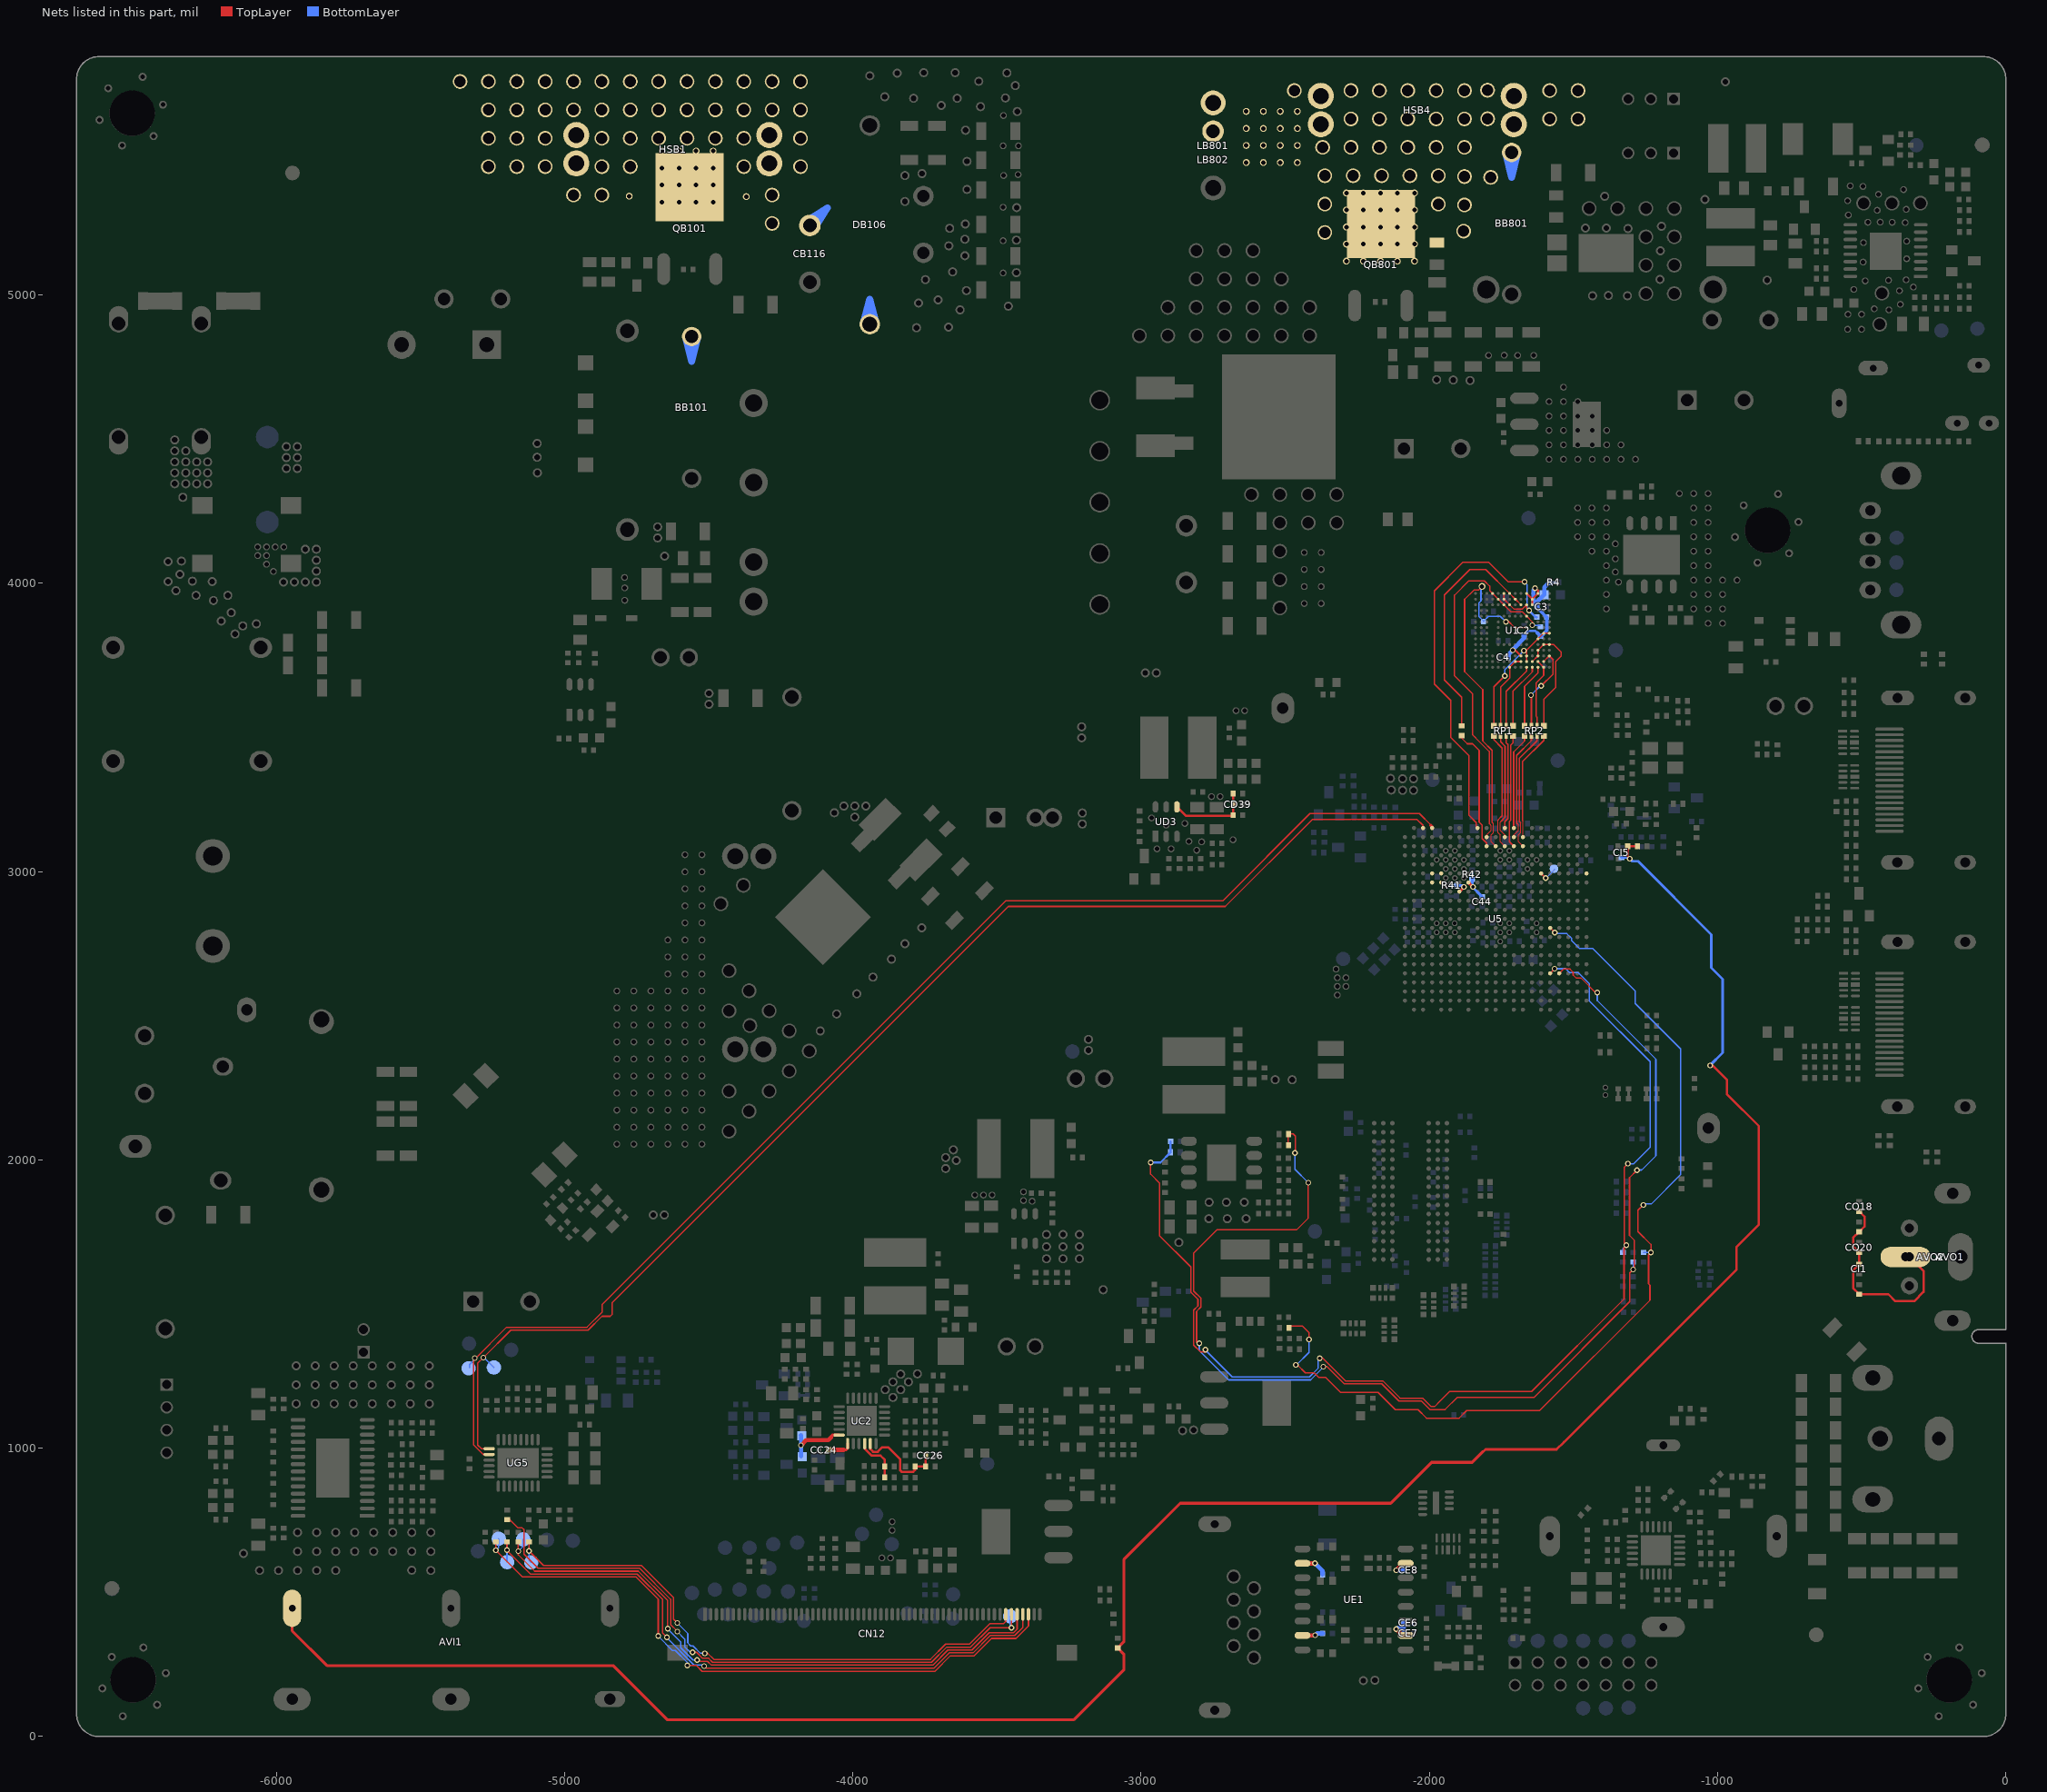
[diagram p0: the nets of this part, all layers, seen from the top]
# Altium PCB MISC84395.PcbDoc (part 12 of 26)
Units mil, origin at the board's own origin, x right, y up, seen from the top; angles counter-clockwise.
Board outline 6692.91 x 5826.77 mil, 2 copper layers (TopLayer, BottomLayer), stack 61.855 mil thick; 951 components, 565 nets, 4374 pads, 1804 vias.
Unrouted connection lines stored in the file: 1.

## Via types
v1: diameter 19.68, hole 11.81, TopLayer to BottomLayer, tented both sides, 1262 vias
v2: diameter 23.62, hole 15.75, TopLayer to BottomLayer, tented both sides, 524 vias
v3: diameter 31.5, hole 19.68, TopLayer to BottomLayer, tented both sides, 11 vias
v4: diameter 24, hole 16, TopLayer to BottomLayer, tented both sides, 6 vias
v5: diameter 19, hole 11.81, TopLayer to BottomLayer, tented both sides, 1 vias

## Nets (pads, with @x,y where several pads share a name; then routed paths per layer and width w, separated by ;. In a path a pad name is that pad's centre, name@x,y a point inside that pad or via, vN(x,y) a via of type N, cw(c..) or ccw(c..) an arc to the next point about the centre after c; other vN are vias at no path point) (continued)
CLK2: CLK2.1 CN12.58 RG89.2 | length 2275.5
  TopLayer w5: RG89.2@-5238.51,674.77 v1(-5238.51,646) -5146.01,553.5 -4752.22,553.5 -4675,476.28 v1(-4675,349) ; v1(-4574,246.5) -4542.76,246.5 -4522.73,226.47 -3715.43,226.47 -3661.66,280.24 -3578.87,280.24 -3518.87,340.24 -3434.26,340.24 -3390.67,383.83 CN12.58@-3390.67,418.08
  BottomLayer w5: v1(-5238.51,646) -5228.26,656.25 CLK2.1@-5228.26,686 ; v1(-4675,349) -4675,347.86 -4626,298.86 -4615.72,298.86 -4574,257.14 v1(-4574,246.5)
CLK3: CLK3.1 CN12.57 RG87.2 | length 2207.6
  TopLayer w5: RG87.2@-5199.51,674.77 v1(-5199.51,647) -5199.51,645.25 -5117.76,563.5 -4748.07,563.5 -4659.34,474.77 -4659.34,358.34 v1(-4645,344) ; v1(-4515.55,243.82) -4509.24,237.5 -4483,237.5 ; -4494.51,237.5 -4483,237.5 ; CN12.57@-3410.35,418.08 -3410.35,378.29 -3438.4,350.24 -3500.5,350.24 -3523.01,350.24 -3583.01,290.24 -3665.8,290.24 -3718.54,237.5 -4483,237.5
  BottomLayer w5: CLK3.1@-5199.51,605.25 v1(-5199.51,647) ; v1@-4645.86,343.14 -4550.96,248.24 -4519.97,248.24 v1(-4515.55,243.82)
CLK4: CLK4.1 CN12.56 RG85.2 | length 2146.6
  TopLayer w5: RG85.2@-5160.51,674.77 v1(-5160.51,643) -5160.51,630.25 -5103.76,573.5 -4743.93,573.5 -4642,471.57 v1(-4642,374) ; v1(-4540.13,265.58) -4535.71,261.16 -4504.02,261.16 -4490.36,247.5 -3722.68,247.5 -3669.94,300.24 -3587.15,300.24 -3527.15,360.24 -3442.54,360.24 -3430.04,372.74 -3430.04,374.5 CN12.56@-3430.04,418.08
  BottomLayer w5: v1(-5160.51,643) -5143.26,660.25 CLK4.1@-5143.26,684 ; v1@-4642,372.47 -4597,327.47 -4597,308.42 -4554.16,265.58 v1(-4540.13,265.58)
CLK5: CLK5.1 CN12.55 RG79.1 | length 2201.9
  TopLayer w5: RG79.1@-5199,752.27 -5190.4,752.27 -5162.73,724.59 -5147.56,724.59 -5140.6,717.63 -5140.6,632.34 -5091.76,583.5 -4739.79,583.5 -4632,475.71 -4632,388.53 v1@-4609,365.53 ; v1(-4556.01,291.96) -4541.99,291.96 -4521.18,271.16 -4499.88,271.16 -4486.22,257.5 -3726.83,257.5 -3674.08,310.24 -3591.3,310.24 -3523.95,377.59 v1(-3449.72,377.59) CN12.55@-3449.72,418.08
  BottomLayer w5: v1(-4609,364) -4582.34,337.34 -4582.34,310.34 -4563.96,291.96 v1(-4556.01,291.96) ; CLK5.1@-3454,417 -3454,381.86 v1(-3449.72,377.59)
CLK6: CLK6.1 CN12.54 RG80.1 | length 2026.6
  TopLayer w5: RG80.1@-5123.26,675.27 v1(-5123.26,644) -5072.76,593.5 -4733.36,593.5 -4622,482.14 -4622,407 v1(-4609,394) ; v1(-4513.5,288.5) -4503.08,288.5 -4482.08,267.5 -3730.97,267.5 -3678.22,320.24 -3595.44,320.24 -3524.34,391.34 -3477.57,391.34 -3469.41,399.5 CN12.54@-3469.41,423.98
  BottomLayer w5: v1(-5123.26,644) -5123.26,612 CLK6.1@-5115.26,604 ; v1(-4609,394) -4572.34,357.34 -4572.34,324.82 -4562.18,314.66 -4554.18,314.66 -4528.03,288.5 v1(-4513.5,288.5)
COAX: AVO1.1 AVO2.2 CI1.2 CO18.2 CO20.2 DO7.K RI1.2 | length 725.7
  TopLayer w8: CO18.2@-508.99,1821.53 -490.16,1802.7 -490.16,1769.38 RI1.2@-509,1750.54 -530,1729.53 -530,1700.54 CO20.2@-508.99,1679.53 CI1.2@-509.01,1638.44 -530,1617.44 -530,1555 DO7.K@-509,1534 -408,1534 -384,1510 -318,1510 -286,1542 -286,1614.74 AVO2.2@-334.65,1663.39
CORE_EN: CD39.1 RD26.1 RD27.1 UD3.4 | length 286.6
  TopLayer w8: UD3.4@-2875.6,3221.6 UD3.4@-2875.6,3224.37 -2845.23,3194 -2682.89,3194 RD27.1@-2681.02,3195.87 ; RD27.1@-2681.65,3196.5 RD27.1@-2681.02,3195.87 ; RD26.1@-2681.02,3270.87 RD27.1@-2681.02,3195.87
CPV1: CPV1.1 U5.AA19 UG5.9 | length 4481.6
  TopLayer w5: UG5.9@-5261.39,998.21 -5288.21,998.21 -5301,1011 -5301,1295 v1(-5281.59,1314.41) -5186.5,1409.5 -4918.15,1409.5 -4870.15,1457.5 -4841.64,1457.5 -4835,1464.14 -4835,1505 -3461,2879 -2708,2879 -2406,3181 -2042.97,3181 -2021.94,3159.96 U5.AA19@-2021.94,3151.04
  BottomLayer w5: v1(-5281.59,1314.41) -5279.41,1314.41 CPV1.1@-5245,1280
CPV2: CPV2.1 U5.AA18 UG5.10 | length 4558.5
  TopLayer w5: UG5.10@-5261.39,978.53 -5282.67,978.53 -5315,1010.86 -5315,1305.53 -5201.03,1419.5 -4922.29,1419.5 -4869.84,1471.95 -4869.84,1498.44 -4867.28,1501 -3469.28,2899 -2716.28,2899 -2414.28,3201 -2034.69,3201 -1994.48,3160.79
  TopLayer w10: -1995.15,3160.12 -1990.44,3155.41 U5.AA18@-1990.44,3151.04
  BottomLayer w5: CPV2.1@-5330,1279 -5330,1290 v1@-5311.47,1308.53 ; v1(-5311.47,1313) v1@-5311.47,1308.53 ; v1@-5307,1313 v1@-5311.47,1308.53
CRD: CE8.1 UE1.7 | length 70.1
  TopLayer w15: v1(-2115,577) -2091.29,600.71 UE1.7@-2081.96,600.71
  BottomLayer w15: v1@-2114,577 v1(-2115,577) CE8.1@-2088.73,577
CRX: RE1.2 UE1.10 | length 93.5
  TopLayer w15: UE1.10@-2440.23,600.71 -2397.23,600.71 v1(-2396.83,601.11)
  BottomLayer w15: v1(-2396.83,601.11) -2370.73,575.01 RE1.2@-2370.73,562
CTD: CE6.2 CE7.2 UE1.2 | length 114.3
  TopLayer w15: v1@-2115.57,370.57 v1@-2115.57,371.97 ; v1(-2115,373) -2092.71,350.71 UE1.2@-2081.96,350.71 UE1.2@-2095.71,350.71
  BottomLayer w15: v1@-2109.53,377 -2088.67,377 ; CE7.2@-2088.67,358.94 -2088.67,377 ; CE6.2@-2088.67,394.94 -2088.67,377
CTX: RE2.2 UE1.15 | length 73.5
  TopLayer w15: UE1.15@-2440.23,350.71 -2396.29,350.71 v1(-2396,351)
  BottomLayer w15: v1(-2396,351) -2389,358 RE2.2@-2369.73,358
CVBS_IN: AVI1.1 CI5.2 DI1.K RI4.2 RI5.2 | length 7894.6
  TopLayer w8: -1813.46,987.49 -1805.11,995.84 -1559.1,995.84 -1533.22,1021.73 -934.5,1620.44 -934.5,1698.07 -857,1775.57 -857,2117 -967.16,2227.16 -967.16,2276.77 -1017.7,2327.31 v1(-1025.96,2327.31)
  TopLayer w9: RI4.2@-1311.91,3087.74 -1311.91,3052.01 v1(-1304.65,3044.74) ; RI4.2@-1310.91,3087.74 RI5.2@-1285.38,3087.74
  TopLayer w10: AVI1.1@-5944.88,444.88 -5944.88,366.82 -5824.06,246 -4831.79,246 -4644.29,58.5 -3232.5,58.5 -3060,231 -3060,286.27 DI1.K@-3081,307.27 -3080.64,307.27 -3060,327.9 -3060,613.21 -2864.21,809 -2134.28,809 -1992.28,951 -1851.37,951 -1814.17,988.2
  BottomLayer w9: CI5.2@-1333.65,3048.74 v1@-1308.65,3048.74 ; v1(-1304.65,3044.74) -1295.62,3035.71 -1276.13,3035.71 -1021.84,2781.42 -1021.84,2666.05 -982.8,2627.01 -982.8,2371.2 -1025.96,2328.04 v1(-1025.96,2327.31)
CVBS_OUT_IC: "CVBS OUT.1" U5.T6 | length 66.2
  TopLayer w5: U5.T6@-1612.49,2993.56 v1(-1596.5,2977.57) -1595.9,2976.98 v1@-1595.9,2976.77
  BottomLayer w5: v1@-1595.9,2976.77 -1565.79,3006.88
D_QB101: BB101.1 CB116.2 DB106.A HSB1.1 HSB1.2 HSB1.3 HSB1.4 pad.VIA5@-4181.39,5444.82 pad.VIA5@-4181.39,5543.25 pad.VIA5@-4181.39,5641.67 pad.VIA5@-4181.39,5740.1 pad.VIA5@-4279.81,5247.97 pad.VIA5@-4279.81,5346.4 pad.VIA5@-4279.81,5641.67 pad.VIA5@-4279.81,5740.1 pad.VIA5@-4369.66,5340.71 pad.VIA5@-4378.24,5444.82 pad.VIA5@-4378.24,5543.25 pad.VIA5@-4378.24,5641.67 pad.VIA5@-4378.24,5740.1 pad.VIA5@-4476.66,5543.25 pad.VIA5@-4476.66,5641.67 pad.VIA5@-4476.66,5740.1 pad.VIA5@-4484.49,5321.71 pad.VIA5@-4484.49,5380.76 pad.VIA5@-4484.49,5439.82 pad.VIA5@-4484.49,5498.87 pad.VIA5@-4543.55,5321.71 pad.VIA5@-4543.55,5380.76 pad.VIA5@-4543.55,5439.82 pad.VIA5@-4543.55,5498.87 pad.VIA5@-4575.09,5543.25 pad.VIA5@-4575.09,5641.67 pad.VIA5@-4575.09,5740.1 pad.VIA5@-4602.6,5321.71 pad.VIA5@-4602.6,5380.76 pad.VIA5@-4602.6,5439.82 pad.VIA5@-4602.6,5498.87 pad.VIA5@-4661.66,5321.71 pad.VIA5@-4661.66,5380.76 pad.VIA5@-4661.66,5439.82 pad.VIA5@-4661.66,5498.87 pad.VIA5@-4673.51,5543.25 pad.VIA5@-4673.51,5641.67 pad.VIA5@-4673.51,5740.1 pad.VIA5@-4771.94,5444.82 pad.VIA5@-4771.94,5543.25 pad.VIA5@-4771.94,5641.67 pad.VIA5@-4771.94,5740.1 pad.VIA5@-4775.66,5342.71 pad.VIA5@-4870.36,5346.4 pad.VIA5@-4870.36,5444.82 pad.VIA5@-4870.36,5543.25 pad.VIA5@-4870.36,5641.67 pad.VIA5@-4870.36,5740.1 pad.VIA5@-4968.79,5346.4 pad.VIA5@-4968.79,5641.67 pad.VIA5@-4968.79,5740.1 pad.VIA5@-5067.21,5444.82 pad.VIA5@-5067.21,5543.25 pad.VIA5@-5067.21,5641.67 pad.VIA5@-5067.21,5740.1 pad.VIA5@-5165.64,5444.82 pad.VIA5@-5165.64,5543.25 pad.VIA5@-5165.64,5641.67 pad.VIA5@-5165.64,5740.1 pad.VIA5@-5264.06,5444.82 pad.VIA5@-5264.06,5543.25 pad.VIA5@-5264.06,5641.67 pad.VIA5@-5264.06,5740.1 pad.VIA5@-5362.49,5740.1 QB101.D
D_QB801: BB801.1 CB809.2 HSB4.1 HSB4.2 HSB4.3 HSB4.4 LB801.2 LB802.2 pad.VIA5@-1484.4,5610.26 pad.VIA5@-1484.4,5708.68 pad.VIA5@-1582.83,5610.26 pad.VIA5@-1582.83,5708.68 pad.VIA5@-1787.1,5407.61 pad.VIA5@-1797.8,5610.8 pad.VIA5@-1798.3,5709.9 pad.VIA5@-1878.1,5312.09 pad.VIA5@-1878.1,5410.51 pad.VIA5@-1878.1,5511.83 pad.VIA5@-1878.1,5610.26 pad.VIA5@-1878.1,5708.68 pad.VIA5@-1881,5221.09 pad.VIA5@-1969.1,5314.98 pad.VIA5@-1969.1,5413.41 pad.VIA5@-1976.53,5511.83 pad.VIA5@-1976.53,5610.26 pad.VIA5@-1976.53,5708.68 pad.VIA5@-2051.84,5117.37 pad.VIA5@-2051.84,5176.43 pad.VIA5@-2051.84,5235.48 pad.VIA5@-2051.84,5294.54 pad.VIA5@-2051.84,5353.59 pad.VIA5@-2067.53,5413.41 pad.VIA5@-2074.95,5511.83 pad.VIA5@-2074.95,5610.26 pad.VIA5@-2074.95,5708.68 pad.VIA5@-2110.9,5117.37 pad.VIA5@-2110.9,5176.43 pad.VIA5@-2110.9,5235.48 pad.VIA5@-2110.9,5294.54 pad.VIA5@-2110.9,5353.59 pad.VIA5@-2165.95,5413.41 pad.VIA5@-2169.95,5117.37 pad.VIA5@-2169.95,5176.43 pad.VIA5@-2169.95,5235.48 pad.VIA5@-2169.95,5294.54 pad.VIA5@-2169.95,5353.59 pad.VIA5@-2173.38,5511.83 pad.VIA5@-2173.38,5610.26 pad.VIA5@-2173.38,5708.68 pad.VIA5@-2229.01,5117.37 pad.VIA5@-2229.01,5176.43 pad.VIA5@-2229.01,5235.48 pad.VIA5@-2229.01,5294.54 pad.VIA5@-2229.01,5353.59 pad.VIA5@-2264.38,5413.41 pad.VIA5@-2271.8,5511.83 pad.VIA5@-2271.8,5610.26 pad.VIA5@-2271.8,5708.68 pad.VIA5@-2288.06,5117.37 pad.VIA5@-2288.06,5176.43 pad.VIA5@-2288.06,5235.48 pad.VIA5@-2288.06,5294.54 pad.VIA5@-2288.06,5353.59 pad.VIA5@-2362.8,5216.56 pad.VIA5@-2362.8,5314.98 pad.VIA5@-2362.8,5413.41 pad.VIA5@-2370.23,5511.83 pad.VIA5@-2457.84,5459.37 pad.VIA5@-2457.84,5518.43 pad.VIA5@-2457.84,5577.48 pad.VIA5@-2457.84,5636.54 pad.VIA5@-2468.65,5708.68 pad.VIA5@-2516.9,5459.37 pad.VIA5@-2516.9,5518.43 pad.VIA5@-2516.9,5577.48 pad.VIA5@-2516.9,5636.54 pad.VIA5@-2575.95,5459.37 pad.VIA5@-2575.95,5518.43 pad.VIA5@-2575.95,5577.48 pad.VIA5@-2575.95,5636.54 pad.VIA5@-2635.01,5459.37 pad.VIA5@-2635.01,5518.43 pad.VIA5@-2635.01,5577.48 pad.VIA5@-2635.01,5636.54 QB801.D
DCDC_SCL_IC: D11.K RD19.2 RT34.1 U5.E5 | length 4090.3
  TopLayer w5: v1(-2967,1991) -2967,1950.8 -2936.5,1920.3 -2936.5,1737.5 -2827.5,1628.5 -2827.5,1625 ; -2827.5,1586 -2827.5,1625 ; v1(-2777,1342) -2775.5,1340.5 -2775.5,1334.5 -2794.12,1334.5 -2817.5,1357.88 -2817.5,1478.83 -2802.66,1493.67 -2802.66,1516.33 -2827.5,1541.17 -2827.5,1625 ; v1@-2372.65,1315 -2291.26,1233.61 -2161.61,1233.61 -2101.61,1173.61 -2023.13,1173.61 -1993.87,1144.34 -1981.55,1144.34 -1970.66,1155.23 ; -1970.66,1155.45 -1929.47,1196.64 -1645.27,1196.64 -1324.67,1517.24 -1324.67,1696.33 ; U5.E5@-1580.99,2647.11 -1580.74,2647.11 v1@-1566.18,2661.67 ; -1324.17,1711.17 -1324.17,1974.24 v1(-1311.51,1986.9)
  BottomLayer w5: v1(-2777,1342) -2777,1340.47 -2683.53,1247 -2416.14,1247 -2385.34,1277.8 -2385.34,1307.04 v1(-2380.21,1312.18) ; v1(-1565.49,2663.1) -1526.82,2663.1 -1513.73,2650.01 -1483.54,2650.01 -1444.91,2611.37 -1444.91,2551.57 -1234.3,2340.97 -1234.3,2043.74 -1291.14,1986.9 v1(-1311.51,1986.9) ; RT34.1@-1328.82,1678.99 -1328.82,1692.18 v1(-1317,1704)
  BottomLayer w8: v1(-2967,1991) -2932.73,1991 D11.K@-2897.73,2026 ; D11.K@-2897.46,2026.27 RD19.2@-2897.46,2064
DCDC_SDA_IC: D12.K RD18.2 RT36.1 U5.E4 | length 4379.8
  TopLayer w5: v1(-2798,1364) -2804,1364 -2807.5,1367.5 -2807.5,1474.69 -2792.66,1489.53 -2792.66,1520.47 -2817.5,1545.31 -2817.5,1676.76 -2737.11,1757.15 -2460.85,1757.15 -2420,1798 v1(-2420,1921) ; RD18.2@-2488.27,2045 -2488.27,2048.46 -2490,2046.73 -2490,2091.73 D12.K@-2488.27,2090 -2473,2090 -2465,2082 -2465,2023 v1(-2466,2024) ; v1(-2368,1283) -2354.79,1283 -2295.4,1223.61 -2165.75,1223.61 -2105.75,1163.61 -2027.28,1163.61 -1998.01,1134.34 -1945.18,1134.34 -1902.88,1176.64 -1636.98,1176.64 -1305.17,1508.45 -1305.17,1607.83 v1(-1293,1620) ; U5.E4@-1549.05,2647.11 U5.E4@-1549.5,2647.11 -1534.91,2661.69 -1511.96,2661.69 -1501.09,2650.83 -1501.09,2641.07 -1490.22,2630.2 -1473.1,2630.2 v1@-1423.65,2580.74 ; v1@-1289.66,1620 -1289.66,1722.04 -1305.67,1738.06 -1305.67,1938.33 v1(-1280,1964)
  BottomLayer w5: v1(-2798,1364) -2798,1338.47 -2696.53,1237 -2412,1237 -2366,1283 v1@-2367,1284 ; v1(-2466,2024) -2466,1967 v1(-2420,1921) ; v1(-1417.57,2580.74) -1417.57,2552.51 -1214.3,2349.25 -1214.3,2014.17 -1263.47,1965 v1@-1279,1965 ; v1@-1292.83,1620.17 RT36.1@-1292.83,1645.52
DDR_EN_IC: R30.2 RD3.2 U5.K5 | length 3335.2
  TopLayer w5: RD3.2@-2487,1417.26 -2480.92,1423.34 -2440.52,1423.34 -2417,1399.83 v1@-2417,1377.79 ; v1(-2463,1289) -2457.53,1289 -2430.34,1261.82 -2399.63,1261.82 -2383.47,1245.66 -2359.87,1245.66 -2307.82,1193.61 -2178.18,1193.61 -2118.18,1133.61 -2039.7,1133.61 -2010.44,1104.34 -1896.72,1104.34 -1870.72,1130.34 -1617.64,1130.34 -1234.96,1513.02 -1234.96,1565.22 -1239.66,1569.92 -1239.66,1670.29 v1(-1231.32,1678.64) -1231.32,1706.79 -1276.17,1751.65 -1276.17,1825.83 v1(-1258,1844) ; U5.K5@-1580.99,2808.97 U5.K5@-1580.99,2804.59 v1@-1565,2788.6
  BottomLayer w5: v1(-2463,1289) -2461,1289 -2417.57,1332.43 v1(-2417.57,1377.22) ; v1@-1561.57,2784.69 -1522.91,2784.69 -1506.89,2768.67 -1506.89,2760.55 -1479.35,2733.01 -1433.29,2733.01 -1286.3,2586.02 -1286.3,2542.87 -1128.3,2384.87 -1128.3,1949.16 -1230.47,1847 v1@-1255,1847 ; R30.2@-1257,1678.84 -1256.79,1678.64 v1(-1231.32,1678.64)
  other v1: -1565.24,2788.36
DRVN: CC24.1 UC2.7 | length 92.9
  TopLayer w10: -4040.14,994 -4032,994 -4024,994 -4017.95,1000.05 UC2.7@-4017.95,1016.18
  TopLayer w15: CC24.1@-4084.11,994 -4032,994
DRVP: CC27.2 CC31.2 UC2.6 | length 224.6
  TopLayer w10: -4078.17,1038.45 -4070.91,1045.71 UC2.6@-4047.48,1045.71
  TopLayer w15: v1(-4180,1010) -4161.5,1028.5 -4084.58,1028.5 -4076.4,1036.68
  BottomLayer w15: CC31.2@-4180,1044.38 CC31.2@-4179.5,1044.88 ; CC27.2@-4179,972 -4179,1044.38 CC31.2@-4179.5,1044.88 ; CC31.2@-4179.5,1044.88 -4179,1045.38 -4180,1045.38 CC31.2@-4179.5,1044.88
DVDD_DDR_RX_0: R41.2 R41.3 U5.P15 | length 48.6
  TopLayer w10: U5.P15@-1895.95,2930.57 v1@-1881.82,2944.71
  BottomLayer w10: R41.2@-1905.75,2951.72 -1887.07,2951.72 v1@-1880.06,2944.71
  other v1: -1880.45,2946.56
DVDD_DDR_RX_1: C44.2 R42.2 R42.3 U5.R14 | length 97.7
  TopLayer w10: U5.R14@-1864.46,2962.07 -1849.48,2947.09 v1@-1849.48,2946.72
  BottomLayer w10: v1@-1851.48,2946.72 R42.2@-1851.48,2972.99 R42.2@-1851.48,2974.99 ; v1@-1849.48,2946.72 -1849.48,2945.31 C44.2@-1816.64,2912.48
  other v1: -1848.95,2946.56
EMMC_CLK: R5.1 U1.M6 U1.N7 U1.P8 | length 831.4
  TopLayer w5: R5.1@-1887.71,3505.08 -1887.71,3604.58 -1947.71,3664.58 -1947.71,3959.04 -1859.4,4047.34 -1804.54,4047.34 U1.P8@-1721.71,3964.51 U1.N7@-1702.02,3944.82 U1.M6@-1682.34,3925.14
EMMC_CLK_IC: R5.2 U5.W12 | length 432.5
  TopLayer w5: R5.2@-1893.71,3471.61 -1893.71,3468.33 -1868.63,3443.25 -1850.28,3443.25 -1827.47,3420.44 -1827.47,3171.34 -1817.21,3161.08 -1817.21,3114.67 -1801.46,3098.92 U5.W12@-1801.46,3088.05
EMMC_CMD_IC: R9.1 U1.M5 U1.M8 U1.N9 U1.P9 U5.AA13 | length 1552.1
  TopLayer w5: U5.AA13@-1832.96,3151.04 -1837.47,3155.55 -1837.47,3170.06 -1862.16,3194.75 -1862.16,3401.2 -1926.05,3465.09 -1926.05,3593.42 -1982.71,3650.08 -1982.71,3973.54 -1883.9,4072.34 -1794.19,4072.34 -1726.58,4004.74 v1(-1669.65,4004.74) ; U1.P9@-1741.39,3964.51 U1.N9@-1741.39,3944.82 U1.M8@-1721.71,3925.14 -1707.41,3910.84 -1676.95,3910.84 U1.M5@-1662.65,3925.14 -1662.65,3913.79 v1(-1654.21,3905.34)
  BottomLayer w5: v1@-1670.65,4004.74 -1661.65,3995.74 -1661.65,3912.78 v1(-1654.21,3905.34) v1@-1655.71,3905.34
  BottomLayer w8: v1(-1654.21,3905.34) -1631.6,3882.74 R9.1@-1627.38,3882.74
EMMC_D0: RP2.7 U1.A3 | length 222.8
  TopLayer w5: RP2.7@-1669.67,3505.06 -1669.67,3642.45 -1623.28,3688.84 U1.A3@-1623.28,3708.6
EMMC_D0_IC: RP2.8 U5.AA9 | length 334.4
  TopLayer w5: U5.AA9@-1706.98,3151.04 -1707.47,3151.54 -1707.47,3415.08 -1669.67,3452.88 RP2.8@-1669.67,3469.63
EMMC_D1: RP1.1 U1.A4 | length 231.1
  TopLayer w5: RP1.1@-1709.59,3505.06 -1709.59,3625.8 -1642.97,3692.42 U1.A4@-1642.97,3708.6
EMMC_D1_IC: RP1.2 U5.W9 | length 393.5
  TopLayer w5: RP1.2@-1709.59,3469.63 -1709.59,3445.97 -1717.47,3438.08 -1717.47,3178.58 -1722.72,3173.33 -1722.72,3103.8 U5.W9@-1706.98,3088.05
EMMC_D2: RP1.3 U1.A5 | length 232.8
  TopLayer w5: RP1.3@-1733.21,3505.06 -1733.21,3624.82 -1662.65,3695.37 U1.A5@-1662.65,3708.6
EMMC_D2_IC: RP1.4 U5.AA10 | length 325.5
  TopLayer w5: U5.AA10@-1738.47,3151.04 -1738.47,3172.58 -1727.47,3183.58 -1727.47,3440.6 -1733.21,3446.34 RP1.4@-1733.21,3469.63
EMMC_D3: RP2.5 U1.B2 U1.C1 | length 310.1
  TopLayer w5: v1(-1647.65,3611.74) -1646.05,3610.14 RP2.5@-1646.05,3505.06 ; v1(-1612,3644) -1571.49,3684.51 -1571.49,3735.55 U1.C1@-1583.91,3747.97 U1.B2@-1603.6,3728.29
  BottomLayer w5: v1(-1647.65,3611.74) -1615.39,3644 v1(-1612,3644)
EMMC_D3_IC: RP2.6 U5.Y9 | length 380.5
  TopLayer w3.94: U5.Y9@-1706.98,3119.55 -1706.98,3127.42 -1691.23,3143.17 -1691.23,3162.34 -1693.97,3165.08
  TopLayer w5: -1693.97,3165.08 -1697.47,3168.58 -1697.47,3403.08 -1646.05,3454.5 RP2.6@-1646.05,3469.63
EMMC_D4: RP2.3 U1.A2 U1.B3 | length 243.9
  TopLayer w5: RP2.3@-1626.37,3505.06 -1626.37,3535.72 -1630.05,3539.4 -1630.05,3653.95 -1603.6,3680.4 U1.A2@-1603.6,3708.6 U1.B3@-1623.28,3728.29
EMMC_D4_IC: RP2.4 U5.W8 | length 418.4
  TopLayer w3.94: -1685.47,3171.58 -1683.35,3169.47 -1683.35,3135.3 -1691.23,3127.42 -1691.23,3103.8 U5.W8@-1675.48,3088.05
  TopLayer w5: -1685.47,3171.58 -1687.47,3173.58 -1687.47,3392.58 -1626.37,3453.69 RP2.4@-1626.37,3469.63
EMMC_D5: RP2.1 U1.B4 U1.C3 U1.D3 U1.E1 U1.E2 | length 428.1
  TopLayer w5: U1.B4@-1642.97,3728.29 U1.C3@-1623.28,3747.97 U1.D3@-1623.28,3767.66 U1.E2@-1603.6,3787.34 U1.E1@-1583.91,3787.34 -1568.68,3787.34 -1542.87,3761.53 -1542.87,3747.16 -1561.49,3728.53 -1561.49,3638.49 -1602.74,3597.24 RP2.1@-1602.74,3505.06
EMMC_D5_IC: RP2.2 U5.Y8 | length 381.9
  TopLayer w3.94: -1677.22,3177.83 -1675.48,3176.08 U5.Y8@-1675.48,3119.55
  TopLayer w5: -1677.22,3177.83 -1677.47,3178.07 -1677.47,3380.58 -1602.74,3455.31 RP2.2@-1602.74,3469.63
EMMC_D6: RP1.7 U1.B5 U1.C5 U1.F3 U1.G1 U1.G2 | length 467.4
  TopLayer w5: RP1.7@-1776.51,3505.06 -1776.51,3640.87 v1(-1738.65,3678.74) ; v1@-1671.21,3767.84 -1662.65,3759.29 ; U1.B5@-1662.65,3728.29 U1.C5@-1662.65,3747.97 -1662.65,3759.29 ; U1.G1@-1583.91,3826.71 U1.G2@-1603.6,3826.71 -1662.65,3767.66 -1662.65,3759.29
  BottomLayer w5: v1(-1738.65,3678.74) -1738.65,3699.93 v1(-1672.5,3766.08) -1669.87,3763.45 -1669.87,3766.5 v1@-1671.21,3767.84
EMMC_D6_IC: RP1.8 U5.W10 | length 409.4
  TopLayer w3.94: -1761.29,3179.77 -1762.09,3178.96 -1762.09,3135.3 -1754.22,3127.42 -1754.22,3103.8 U5.W10@-1738.47,3088.05
  TopLayer w5: RP1.8@-1776.51,3469.63 -1776.51,3457.65 -1747.47,3428.6 -1747.47,3193.58 -1761.29,3179.77
EMMC_D7: RP1.5 U1.A8 U1.B6 U1.B7 | length 264.3
  TopLayer w5: RP1.5@-1752.89,3505.06 -1752.89,3639.97 -1721.3,3671.56 -1721.3,3708.2 U1.A8@-1721.71,3708.6 U1.B7@-1702.02,3728.29 U1.B6@-1682.34,3728.29
EMMC_D7_IC: RP1.6 U5.Y10 | length 369.9
  TopLayer w3.94: -1751.28,3174.77 -1754.22,3171.83 -1754.22,3143.17 -1738.47,3127.42 U5.Y10@-1738.47,3119.55
  TopLayer w5: RP1.6@-1752.89,3469.63 -1752.89,3450.03 -1737.47,3434.6 -1737.47,3188.58 -1751.28,3174.77
EMMC_DS_IC: R11.2 U1.H5 U5.W11 | length 1290.5
  TopLayer w3.94: -1780.13,3168.37 -1777.84,3166.08 -1777.84,3135.3 -1785.72,3127.42 -1785.72,3103.8 U5.W11@-1769.97,3088.05
  TopLayer w5: v2(-1817.48,3988.72) -1829.27,3976.93 -1844.96,3976.93 -1877.71,3944.19 -1877.71,3693.57 -1814.71,3630.57 -1814.71,3452.94 -1782.47,3420.7 -1782.47,3170.71 -1780.13,3168.37 ; v1@-1729.12,3871.23 -1704.29,3846.4 U1.H5@-1662.65,3846.4
  BottomLayer w5: v2@-1820.98,3992.08 -1820.98,3938.34 -1827.74,3931.58 -1827.74,3884.56 -1811.65,3868.47 -1794.72,3885.4 -1753.74,3885.4 v1(-1734.35,3866.01) ; v2@-1820.91,3992.15 -1820.91,3993.54 v2@-1820.21,3992.85
EMMC_RST_IC: R10.1 U1.K5 U1.M9 U1.N10 U1.P11 U5.Y12 | length 1308.4
  TopLayer w3.94: U5.Y12@-1801.46,3119.55 -1801.46,3127.42 -1785.72,3143.17 -1785.72,3160.03 -1788.24,3162.56
  TopLayer w5: -1847.52,3471.61 -1792.47,3416.56 -1792.47,3166.78 -1788.24,3162.56 ; -1838.58,3462.66 -1850.71,3474.8 -1850.71,3617.07 -1912.71,3679.07 -1912.71,3958.68 -1863.36,4008.03 -1808.9,4008.03 -1790.91,3990.05 -1790.91,3974.66 U1.P11@-1780.76,3964.51 U1.M9@-1741.39,3925.14 -1716.6,3900.34 -1677.23,3900.34 U1.K5@-1662.65,3885.77 -1642.65,3865.76 -1642.65,3854.99 v1(-1642.97,3854.66)
  BottomLayer w5: v1(-1642.97,3854.66) -1641.78,3853.47 R10.1@-1615.65,3853.47
EMMC_VIO: C1.2 C2.2 C3.2 C4.2 R4.2 R4.3 R9.2 R10.2 U1.C6 U1.M4 U1.N4 U1.P3 U1.P5 | length 599.9
  TopLayer w7: v1@-1702.21,3767.84 U1.C6@-1682.34,3747.97 ; U1.P5@-1662.65,3964.51 U1.N4@-1642.97,3944.82 ; U1.M4@-1642.97,3925.14 U1.N4@-1642.97,3944.82 ; v1@-1631.21,3982.84 -1623.28,3974.92 U1.P3@-1623.28,3964.51 U1.N4@-1642.97,3944.82
  BottomLayer w8: C2.2@-1671.48,3819.98 -1657.33,3834.14 -1632.33,3834.14 -1625.81,3827.61
  BottomLayer w12: C3.2@-1627.38,3918.74 -1627.38,3917 -1607.52,3897.14 -1607.52,3896.35 R9.2@-1593.91,3882.74 -1592.71,3881.53 -1592.71,3836.15 -1614.85,3814.01 -1615.65,3814.01 -1615.65,3817.45 -1625.81,3827.61
  BottomLayer w15: C4.2@-1726.64,3742.74 -1726.65,3751.91 v1(-1710.71,3767.84) -1710.71,3770.75 -1671.48,3809.97 C2.2@-1671.48,3819.98 ; v1(-1633.21,3982.84) -1639.3,3976.75 -1639.3,3930.67 C3.2@-1627.38,3918.74 -1627.38,3934.82 C1.2@-1601.46,3960.74 -1601.46,3986.01 R4.2@-1584.46,4003
FBN: CC26.1 RC21.1 RC22.2 UC2.11 | length 331.5
  TopLayer w8: UC2.11@-3939.21,1016.18 -3939.21,997.21 -3929.5,987.5 -3913.6,987.5 -3897.91,1003.18 -3877.21,1003.18 -3835.59,961.56 -3835.59,923.43 -3830.32,918.16 -3790.84,918.16 -3784.27,924.73 RC22.2@-3784.27,937 RC21.1@-3747.73,937 CC26.1@-3747.73,975
FBP: RC26.2 RC29.1 UC2.10 | length 163.2
  TopLayer w8: UC2.10@-3958.9,1016.18 -3958.9,998.51 -3934.88,974.5 -3903.5,974.5 -3889.73,960.73 RC29.1@-3889.73,900
FUART_CTS_IC: U5.R17
FUART_RTS_IC: U5.R18
FUART_RXD_IC: U5.T18
FUART_TXD_IC: U5.T17
GIN1M_IN_IC: U5.T1